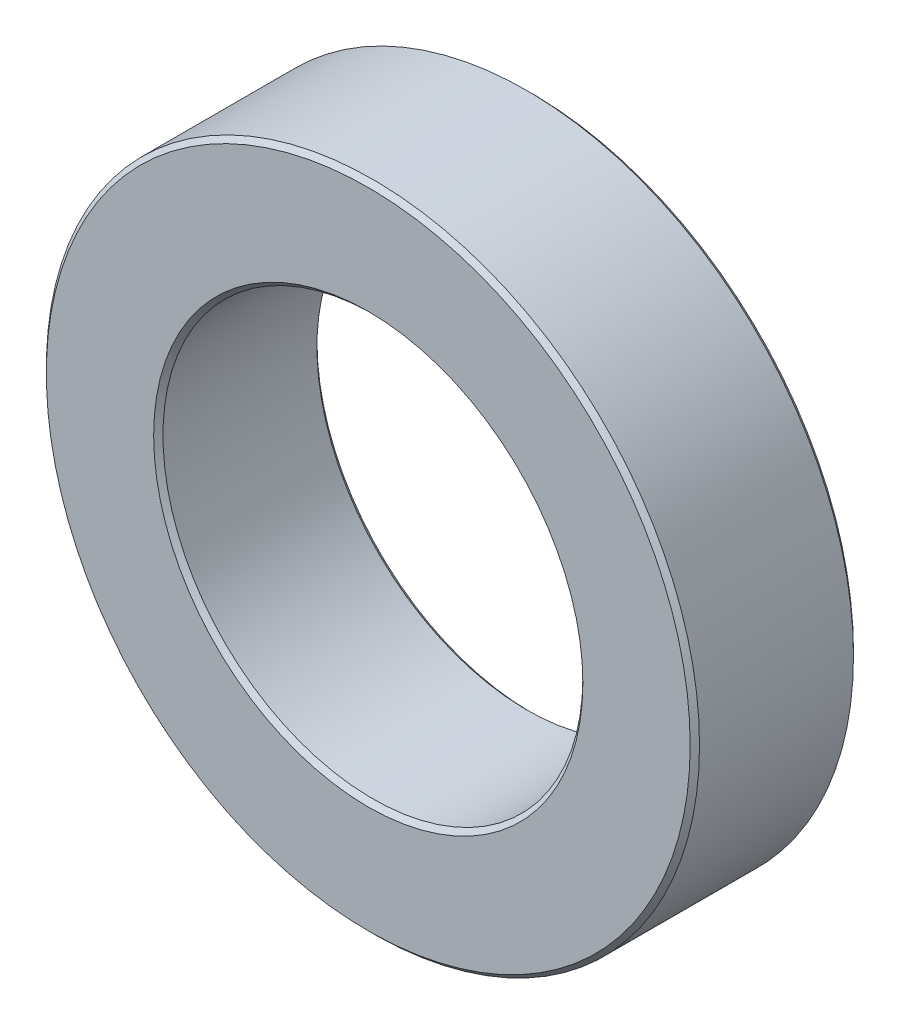
from build123d import *

# Parameters (mm, degrees)
SKETCH_1_R      = 35
SKETCH_1_R_2    = 22.5
EXTRUDE_1_DEPTH = 17.5
CHAMFER_1_SIZE  = 0.5


with BuildPart() as part:
    # 草图1 → 凸台-拉伸1 (new body)
    with BuildSketch(Plane.XY):
        Circle(SKETCH_1_R)
        Circle(SKETCH_1_R_2, mode=Mode.SUBTRACT)
    extrude(amount=EXTRUDE_1_DEPTH)

    # 倒角1
    chamfer_1_edges = [part.edges().sort_by_distance(p)[0] for p in [
        (-35, 0, 0),
        (-35, 0, 17.5),
        (-22.5, 0, 0),
        (-22.5, 0, 17.5),
    ]]
    chamfer(chamfer_1_edges, length=CHAMFER_1_SIZE)


solid = part.part
